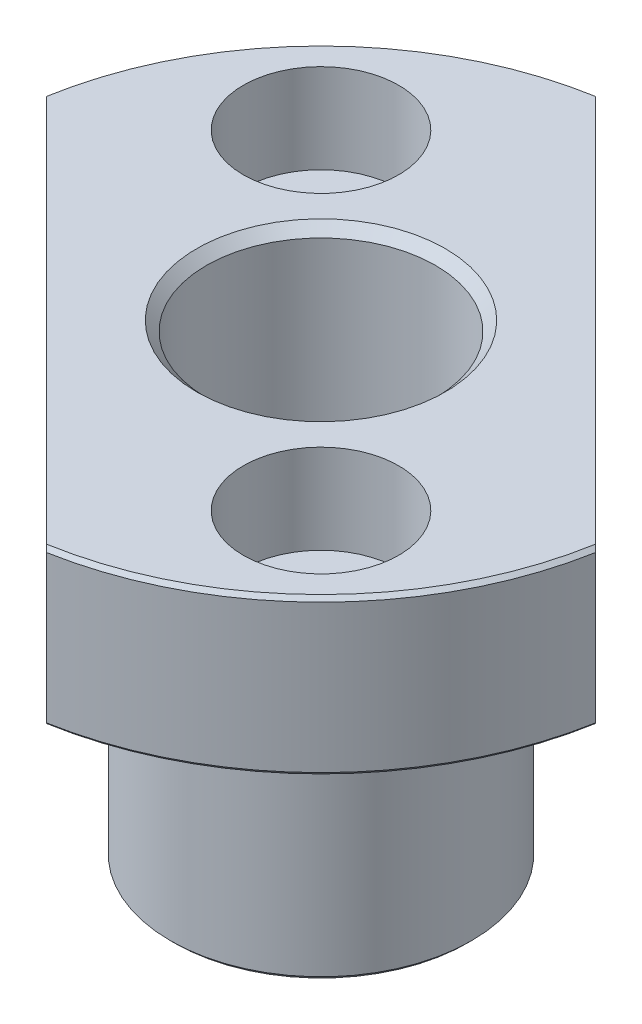
from build123d import *

# Parameters (mm, degrees)
G1_4_TAPPED_HOLE1_D                               = 11.8
HOLE_SIZE_BASED_ON_SOCKET_HEAD_CAP_SC_D           = 4.8
HOLE_SIZE_BASED_ON_SOCKET_HEAD_CAP_SC_CBORE_D     = 8
HOLE_SIZE_BASED_ON_SOCKET_HEAD_CAP_SC_CBORE_DEPTH = 4.6
FILLET1_R                                         = 0.2
CHAMFER1_SIZE                                     = 0.2
CHAMFER2_SIZE                                     = 0.5
CUT_EXTRUDE1_DEPTH                                = 35.474628352


with BuildPart() as part:
    # Sketch2 → Revolve1 (revolve)
    with BuildSketch(Plane.XY, mode=Mode.PRIVATE) as revolve1_sk:
        Polygon((0, 24), (-17.5, 24), (-17.5, 16), (-7.75, 16), (-7.75, 0), (0, 0), align=None)
    revolve(revolve1_sk.sketch.rotate(Axis((0, 0, 0), (0, 1, 0)), 270), axis=Axis((0, 0, 0), (0, 1, 0)))

    # G1/4 Tapped Hole1 (through all)
    with Locations(Plane.ZX.offset(24)):
        with Locations((0, 0)):
            Hole(G1_4_TAPPED_HOLE1_D / 2)

    # Hole Size (% based on) Socket Head Cap Screw Type 1 (through all)
    with Locations(Plane(origin=(-8.485281374, 24, -8.485281374), x_dir=(0, 0, 1), z_dir=(0, 1, 0))):
        with Locations((0, 0), (16.970562748, 16.970562748)):
            CounterBoreHole(HOLE_SIZE_BASED_ON_SOCKET_HEAD_CAP_SC_D / 2, HOLE_SIZE_BASED_ON_SOCKET_HEAD_CAP_SC_CBORE_D / 2, HOLE_SIZE_BASED_ON_SOCKET_HEAD_CAP_SC_CBORE_DEPTH)

    # Fillet1
    fillet1_edges = [part.edges().sort_by_distance(p)[0] for p in [
        (0, 16, 7.75),
    ]]
    fillet(fillet1_edges, radius=FILLET1_R)

    # Chamfer1
    chamfer1_edges = [part.edges().sort_by_distance(p)[0] for p in [
        (0, 0, 7.75),
        (0, 16, 17.5),
        (0, 24, 17.5),
    ]]
    chamfer(chamfer1_edges, length=CHAMFER1_SIZE)

    # Chamfer2
    chamfer2_edges = [part.edges().sort_by_distance(p)[0] for p in [
        (0, 24, 5.9),
        (0, 0, 5.9),
    ]]
    chamfer(chamfer2_edges, length=CHAMFER2_SIZE)

    # Sketch7 → Cut-Extrude1 (cut, through all)
    with BuildSketch(Plane(origin=(0, 24, 0), x_dir=(1, 0, 0), z_dir=(0, 1, 0))):
        with BuildLine():
            Line((2.911166407, -17.053302031), (-17.053302031, 2.911166407))
            ThreePointArc((-17.053302031, 2.911166407), (-12.232947315, -12.232947315), (2.911166407, -17.053302031))
        make_face()
        with BuildLine():
            ThreePointArc((17.3, 0), (11.156317071, 13.222200627), (-2.911166407, 17.053302031))
            Line((-2.911166407, 17.053302031), (17.053302031, -2.911166407))
            ThreePointArc((17.053302031, -2.911166407), (17.238215179, -1.460800272), (17.3, 0))
        make_face()
        with BuildLine():
            Line((-17.053302031, 2.911166407), (-17.226115818, 3.083980194))
            ThreePointArc((-17.226115818, 3.083980194), (-12.374368671, -12.374368671), (3.083980194, -17.226115818))
            Line((3.083980194, -17.226115818), (2.911166407, -17.053302031))
            ThreePointArc((2.911166407, -17.053302031), (-12.232947315, -12.232947315), (-17.053302031, 2.911166407))
        make_face()
        with BuildLine():
            ThreePointArc((17.5, 0), (11.23121424, 13.42050024), (-3.083980194, 17.226115818))
            Line((-3.083980194, 17.226115818), (-2.911166407, 17.053302031))
            ThreePointArc((-2.911166407, 17.053302031), (11.156317071, 13.222200627), (17.3, 0))
            ThreePointArc((17.3, 0), (17.238215179, -1.460800272), (17.053302031, -2.911166407))
            Line((17.053302031, -2.911166407), (17.226115818, -3.083980194))
            ThreePointArc((17.226115818, -3.083980194), (17.431394477, -1.548058977), (17.5, 0))
        make_face()
    extrude(amount=-CUT_EXTRUDE1_DEPTH, mode=Mode.SUBTRACT)


solid = part.part
